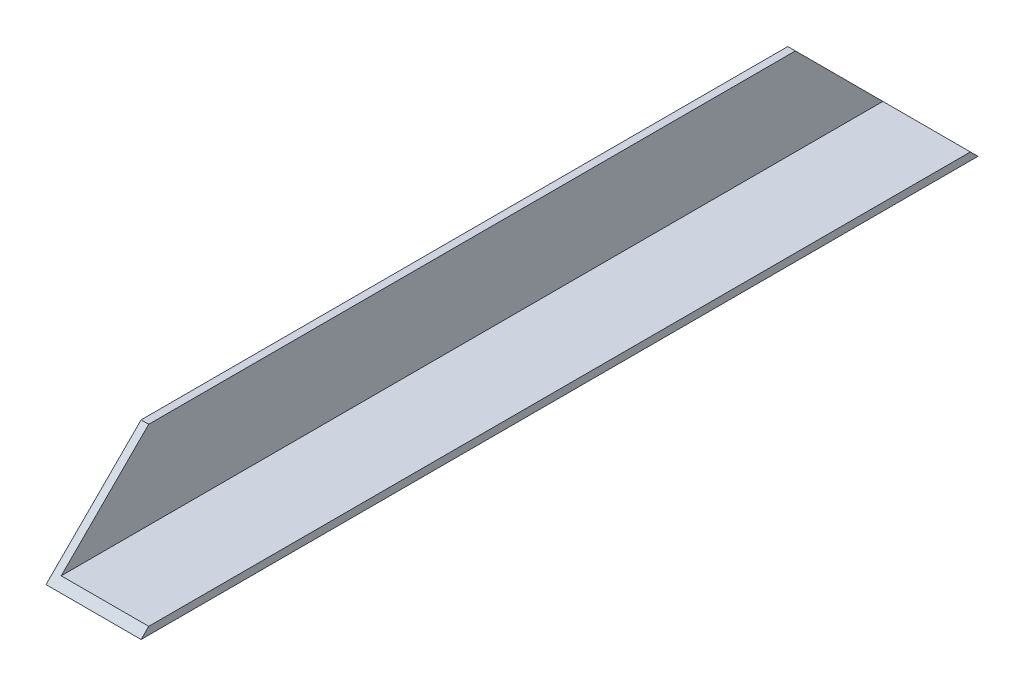
SolidWorks part; units mm, degrees
material "A3"
ref_plane "前视基准面" through (0, 0, 0) normal (0, 0, 1) x (1, 0, 0)
ref_plane "上视基准面" through (0, 0, 0) normal (0, 1, 0) x (1, 0, 0)
ref_plane "右视基准面" through (0, 0, 0) normal (1, 0, 0) x (0, 0, -1)
sketch "草图1" plane through (0, 0, 0) normal (0, 0, 1) x (1, 0, 0)
  line L0 (0, 125) -> (0, 0)
  line L1 (0, 0) -> (125, 0)
  line L2 (125, 0) -> (125, 10)
  line L3 (10, 125) -> (10, 10)
  line L4 (10, 10) -> (125, 10)
  line L5 (0, 125) -> (10, 125)
  dimension "D1" = 125
  dimension "D2" = 10
  dimension "D3" = 10
extrude "凸台-拉伸1" add sketch "草图1" along normal mid plane 1100 contours L5 L0 L1 L2 L4 L3
sketch "草图2" plane through (125, 0, 0) normal (1, 0, 0) x (0, 0, -1)
  line L0 (-550, 0) -> (-550, 125)
  line L1 (-550, 125) -> (-425, 125)
  line L2 (-550, 125) -> (550, 125) construction
  line L3 (-425, 125) -> (-550, 0)
  line L4 (0, 0) -> (0, 125) construction
  line L5 (425, 125) -> (550, 0)
  line L6 (550, 125) -> (425, 125)
  line L7 (550, 0) -> (550, 125)
  dimension "D1" = 45
extrude "切除-拉伸1" cut sketch "草图2" against normal through all
